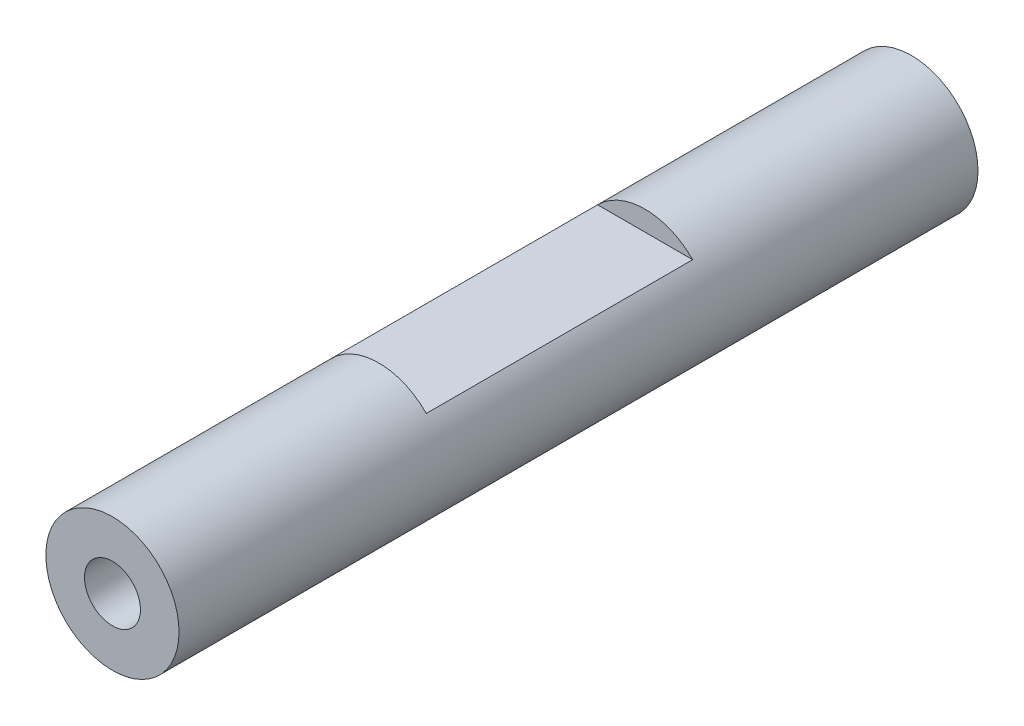
from build123d import *

# Parameters (mm, degrees)
SKETCH1_R                       = 5
BOSS_EXTRUDE1_DEPTH             = 60
SKETCH2_W                       = 20
SKETCH2_H                       = 20
CUT_EXTRUDE1_DEPTH              = 1.5
M5_TAPPED_HOLE1_D               = 4.2
M5_TAPPED_HOLE1_DEPTH           = 15
M5_TAPPED_HOLE1_TIP             = 1.2618073
M5_TAPPED_HOLE1_ON_FACE_2_D     = 4.2
M5_TAPPED_HOLE1_ON_FACE_2_DEPTH = 15
M5_TAPPED_HOLE1_ON_FACE_2_TIP   = 1.2618073


with BuildPart() as part:
    # Sketch1 → Boss-Extrude1 (new body)
    with BuildSketch(Plane.XY):
        with Locations((-90, 55)):
            Circle(SKETCH1_R)
    extrude(amount=BOSS_EXTRUDE1_DEPTH)

    # Sketch2 → Cut-Extrude1 (cut)
    with BuildSketch(Plane(origin=(0, 60, 0), x_dir=(1, 0, 0), z_dir=(0, 1, 0))):
        with Locations((-90, -30)):
            Rectangle(SKETCH2_W, SKETCH2_H)
    cut_extrude1 = extrude(amount=-CUT_EXTRUDE1_DEPTH, mode=Mode.SUBTRACT)

    # Mirror1: Cut-Extrude1 across plane
    add(cut_extrude1.mirror(Plane.ZX.offset(55)), mode=Mode.SUBTRACT)

    # M5 Tapped Hole1
    with Locations(Plane(origin=(-90, 55, 0), x_dir=(-1, 0, 0), z_dir=(0, 0, -1))):
        with Locations((0, 0)):
            Hole(M5_TAPPED_HOLE1_D / 2, depth=M5_TAPPED_HOLE1_DEPTH)
            with Locations((0, 0, -(M5_TAPPED_HOLE1_DEPTH + M5_TAPPED_HOLE1_TIP / 2))):  # 118° drill point
                Cone(0, M5_TAPPED_HOLE1_D / 2, M5_TAPPED_HOLE1_TIP, mode=Mode.SUBTRACT)

    # M5 Tapped Hole1 on face 2
    with Locations(Plane(origin=(-90, 55, 60), x_dir=(1, 0, 0), z_dir=(0, 0, 1))):
        with Locations((0, 0)):
            Hole(M5_TAPPED_HOLE1_ON_FACE_2_D / 2, depth=M5_TAPPED_HOLE1_ON_FACE_2_DEPTH)
            with Locations((0, 0, -(M5_TAPPED_HOLE1_ON_FACE_2_DEPTH + M5_TAPPED_HOLE1_ON_FACE_2_TIP / 2))):  # 118° drill point
                Cone(0, M5_TAPPED_HOLE1_ON_FACE_2_D / 2, M5_TAPPED_HOLE1_ON_FACE_2_TIP, mode=Mode.SUBTRACT)


solid = part.part
